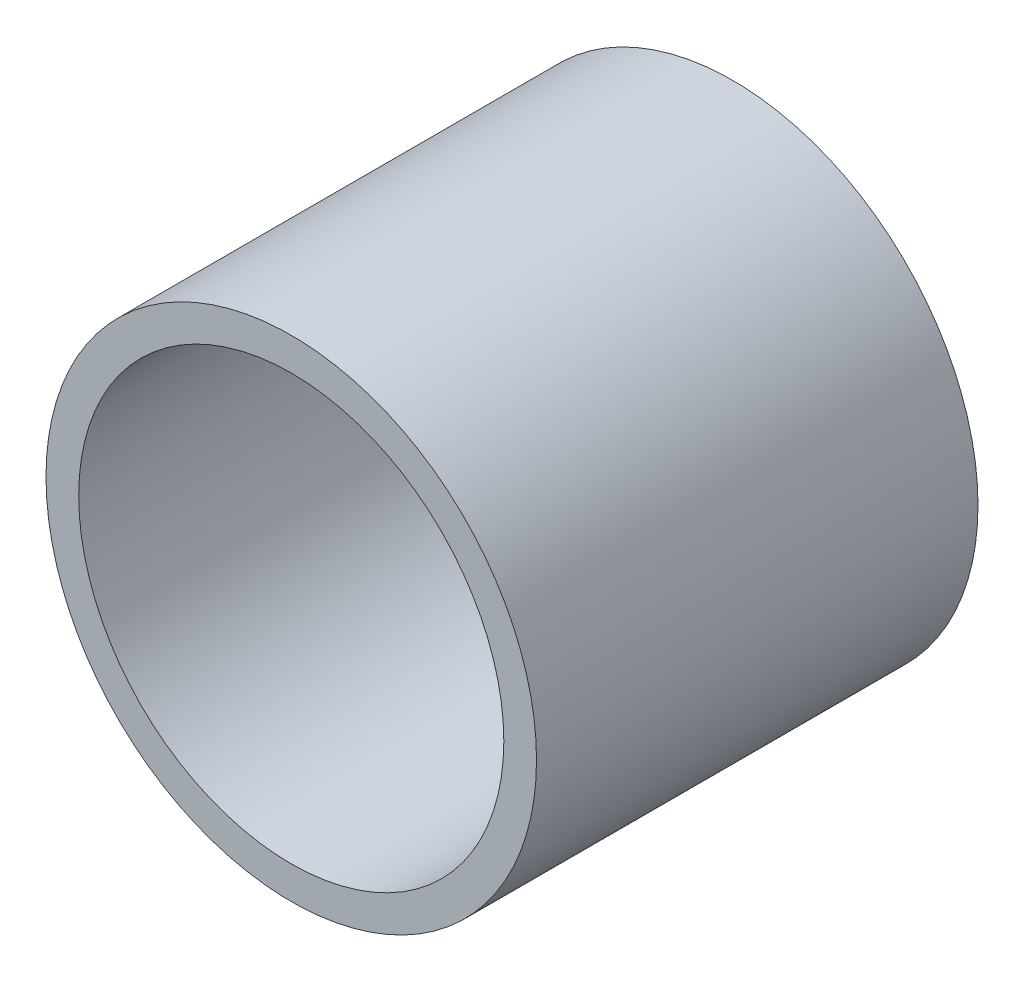
from build123d import *

# Parameters (mm, degrees)
SKETCH1_R           = 15
SKETCH1_R_2         = 13
BOSS_EXTRUDE1_DEPTH = 27


with BuildPart() as part:
    # Sketch1 → Boss-Extrude1 (new body)
    with BuildSketch(Plane.XY):
        Circle(SKETCH1_R)
        Circle(SKETCH1_R_2, mode=Mode.SUBTRACT)
    extrude(amount=BOSS_EXTRUDE1_DEPTH)


solid = part.part
